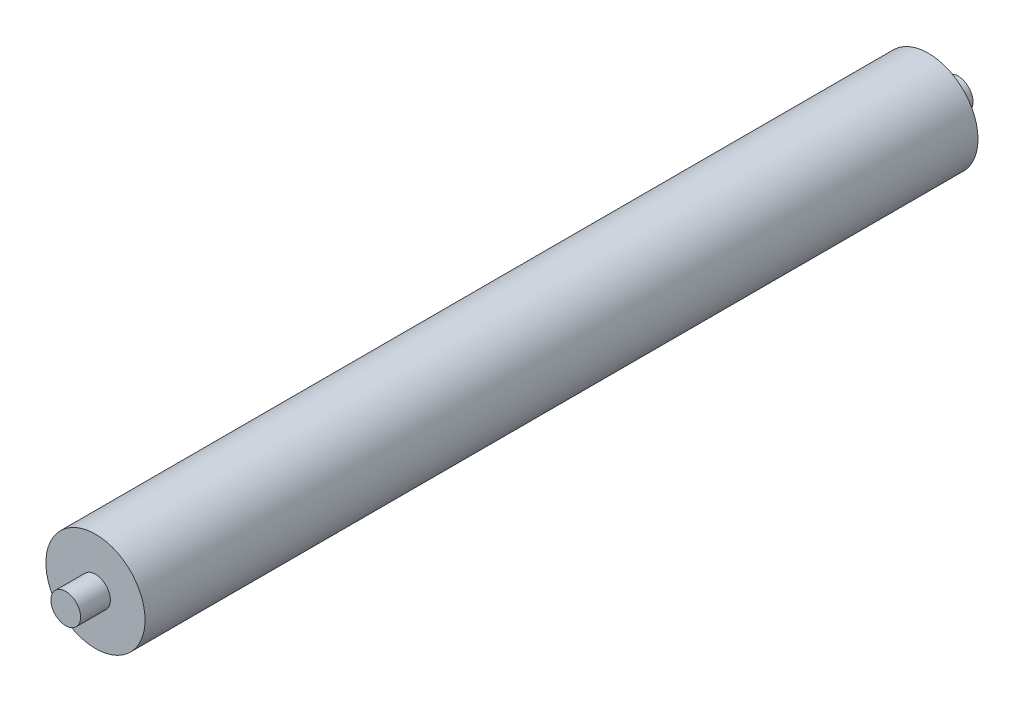
from build123d import *

# Parameters (mm, degrees)
SKETCH_1_R      = 25
EXTRUDE_1_DEPTH = 420
SKETCH_2_R      = 7.5
EXTRUDE_2_DEPTH = 15
EXTRUDE_START   = 15
SKETCH_3_R      = 7.5
EXTRUDE_3_DEPTH = 15


with BuildPart() as part:
    # 草图1 → 凸台-拉伸1 (new body)
    with BuildSketch(Plane.XY):
        Circle(SKETCH_1_R)
    extrude(amount=EXTRUDE_1_DEPTH)

    # 草图2 → 凸台-拉伸2 (add)
    with BuildSketch(Plane.XY.offset(420)):
        Circle(SKETCH_2_R)
    extrude(amount=EXTRUDE_2_DEPTH)

    # 草图3 → 凸台-拉伸3 (add)
    with BuildSketch(Plane(origin=(0, 0, 0), x_dir=(-1, 0, 0), z_dir=(0, 0, -1)).offset(EXTRUDE_START)):
        with Locations(Location((0, 0, 0), (0, 0, 180))):
            Circle(SKETCH_3_R)
    extrude(amount=-EXTRUDE_3_DEPTH)


solid = part.part
